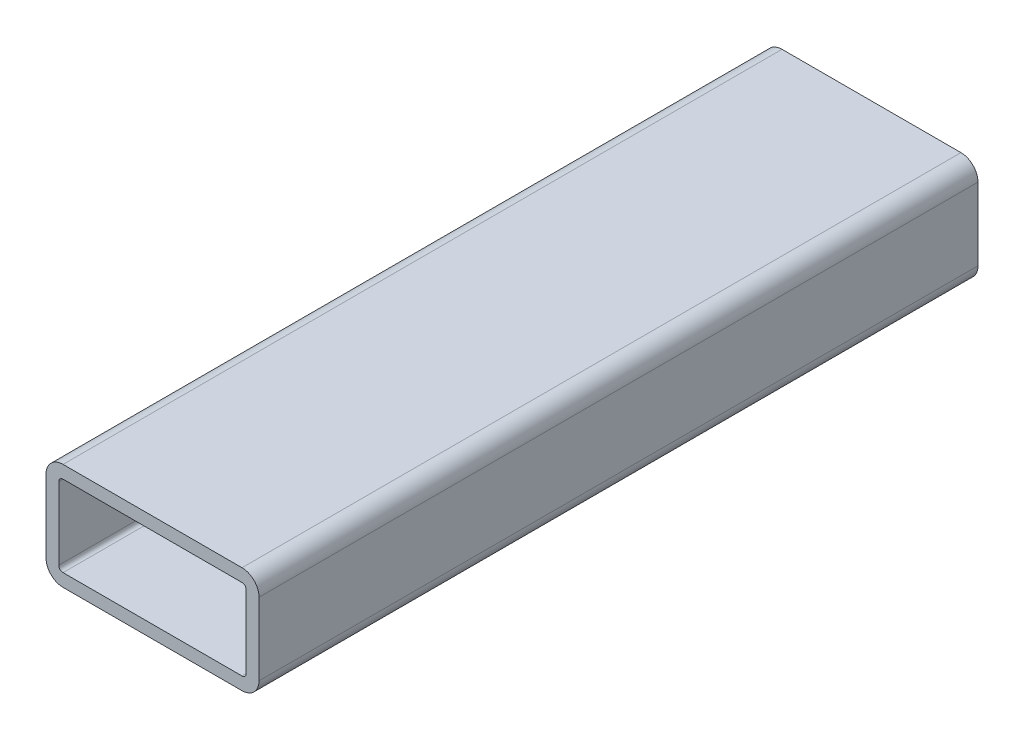
from build123d import *

# Parameters (mm, degrees)
BOSS_EXTRUDE2_DEPTH = 337.5
SHELL1_T            = -6


with BuildPart() as part:
    # Sketch2 → Boss-Extrude2 (new body)
    with BuildSketch(Plane.XY):
        with BuildLine():
            Line((42, 25), (-42, 25))
            ThreePointArc((-42, 25), (-47.656854249, 22.656854249), (-50, 17))
            Line((-50, 17), (-50, -17))
            ThreePointArc((-50, -17), (-47.656854249, -22.656854249), (-42, -25))
            Line((-42, -25), (42, -25))
            ThreePointArc((42, -25), (47.656854249, -22.656854249), (50, -17))
            Line((50, -17), (50, 17))
            ThreePointArc((50, 17), (47.656854249, 22.656854249), (42, 25))
        make_face()
    extrude(amount=BOSS_EXTRUDE2_DEPTH)

    # Shell1
    shell1_openings = [part.faces().sort_by_distance(p)[0] for p in [
        (0, 0, 337.5),
        (0, 0, 0),
    ]]
    offset(amount=SHELL1_T, openings=shell1_openings, kind=Kind.INTERSECTION)


solid = part.part
